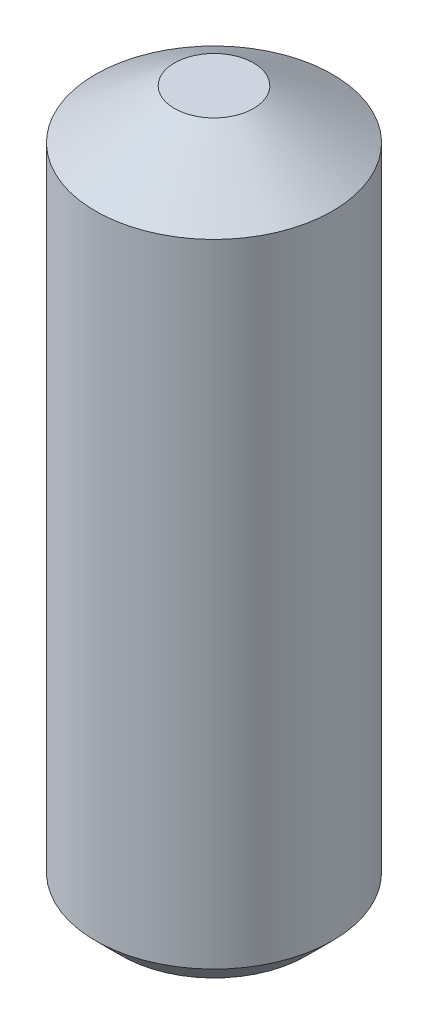
SolidWorks part; units mm, degrees
ref_plane "Front Plane" through (0, 0, 0) normal (0, 0, 1) x (1, 0, 0)
ref_plane "Top Plane" through (0, 0, 0) normal (0, 1, 0) x (1, 0, 0)
ref_plane "Right Plane" through (0, 0, 0) normal (1, 0, 0) x (0, 0, -1)
sketch "Sketch1" plane through (0, 0, 0) normal (0, 0, 1) x (1, 0, 0)
  line L0 (0, 26.8747) -> (1.5, 26.8747)
  line L1 (1.5, 26.8747) -> (4.5002, 25)
  line L2 (4.5002, 25) -> (4.5002, 0)
  line L3 (4.5002, 0) -> (0, 0)
  line L4 (0, 0) -> (0, 26.8747)
  dimension "D1" = 1.5
  dimension "D2" = 58
  dimension "D3" = 25
revolve "Revolve1" add sketch "Sketch1" angle 360 about L4
chamfer "Chamfer1" distance 1 angle 45 1 edges at (4.5002, 0, 0)
